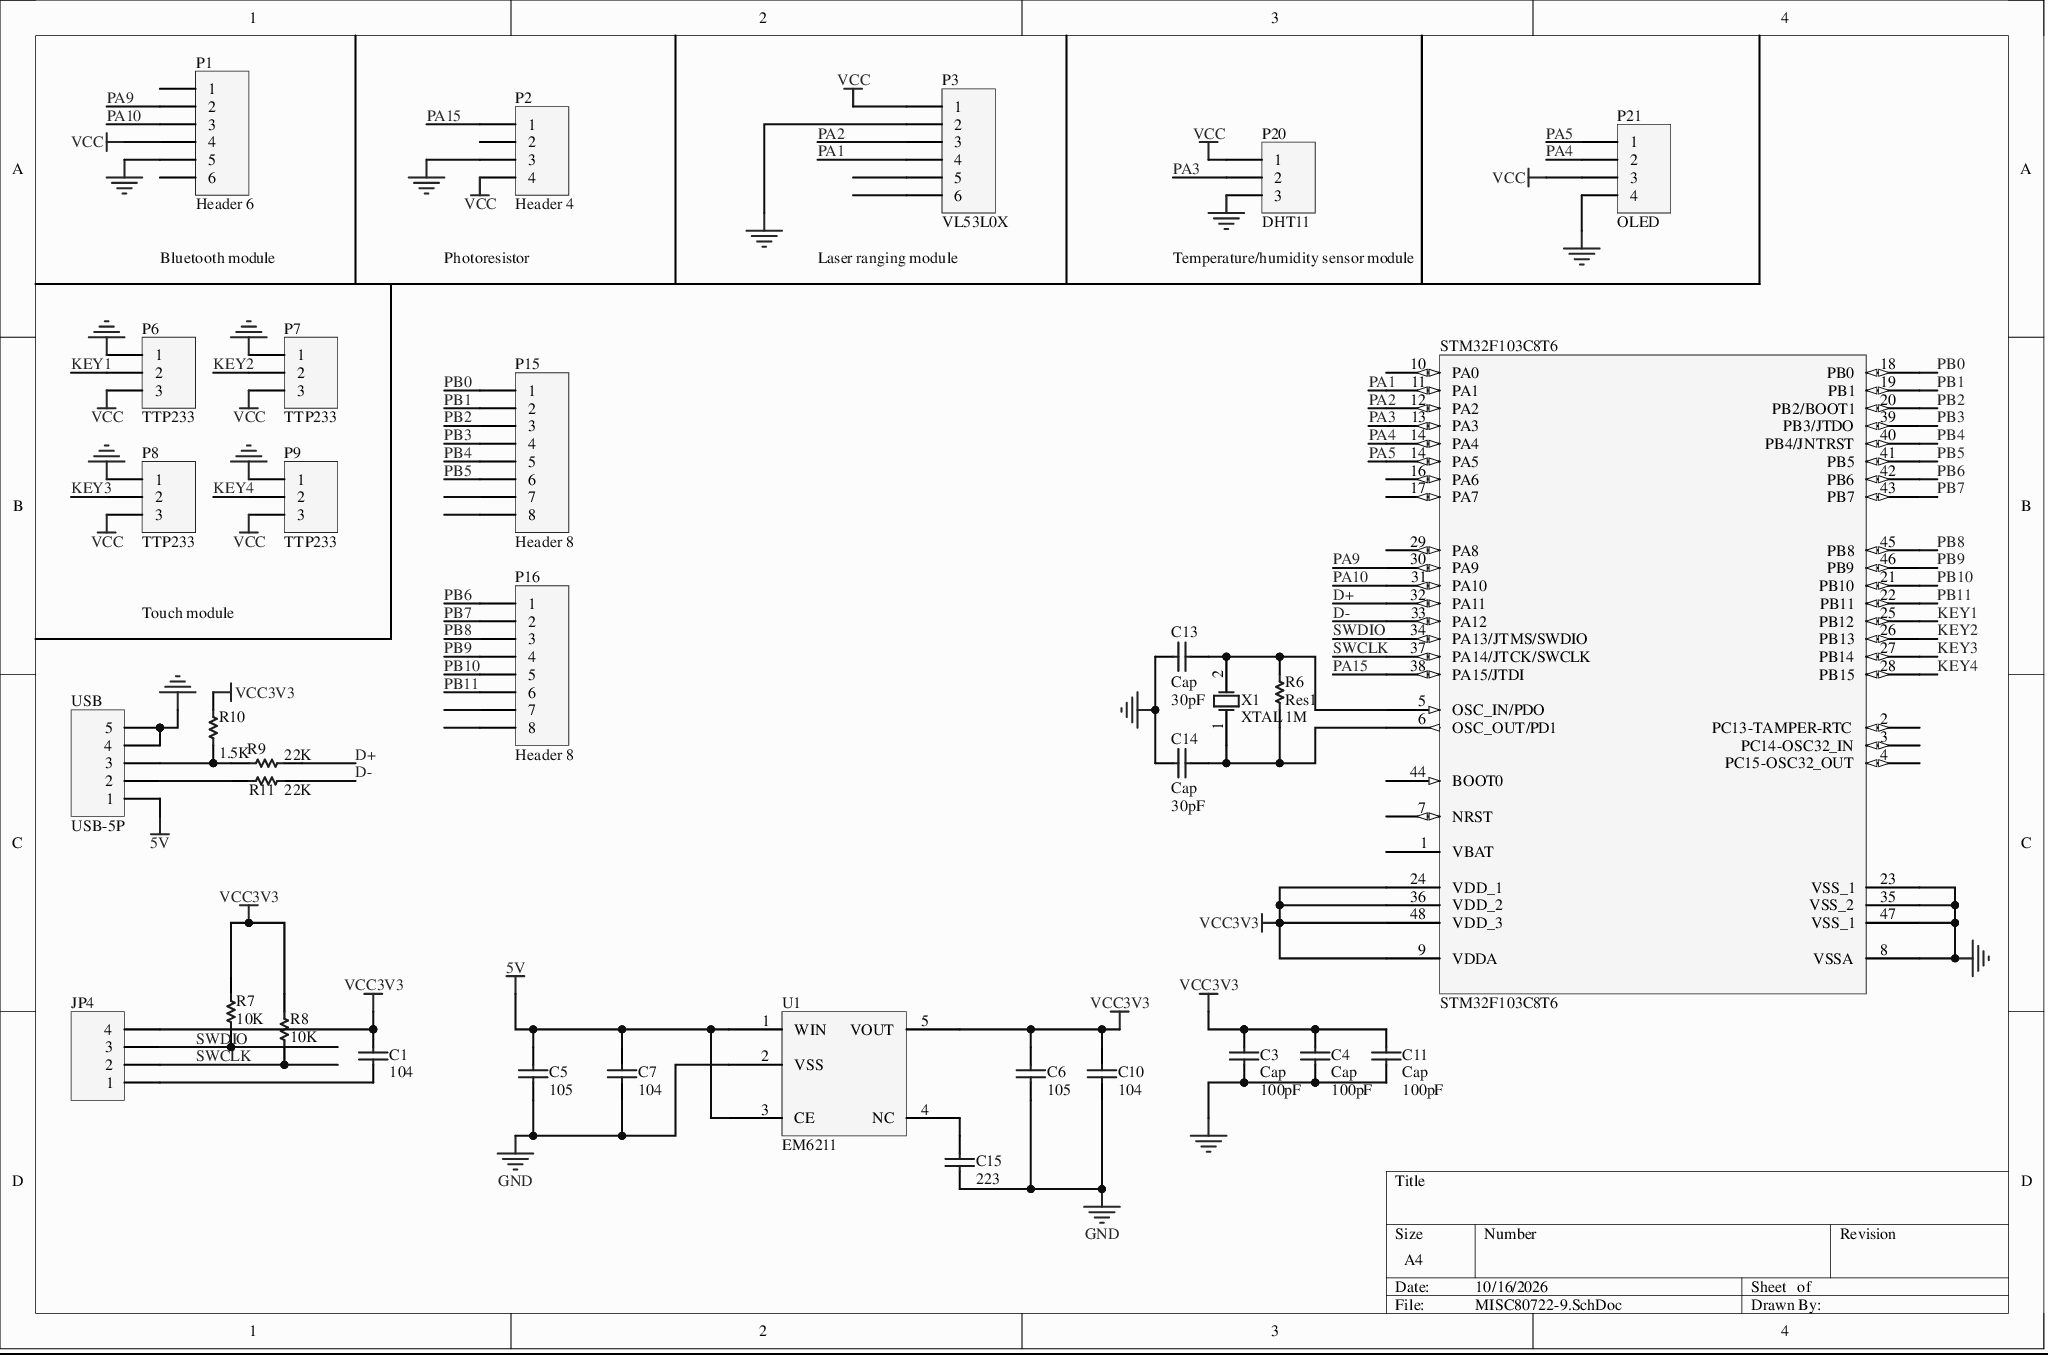
[diagram p0: MISC80722-9.SchDoc]
# Altium project MISC80722-4.PrjPcb
1 sheet, 33 parts. Net scope: global (net labels, ports and power ports of the same name join across sheets).
Board file: MISC80722.PcbDoc

## Sheet MISC80722-9.SchDoc
size A4; SheetNumber: 1; SheetTotal: 1

### Parts
C1  104  [RAD-0.3]
C3  Cap  value 100pF  [RAD-0.3]
C4  Cap  value 100pF  [RAD-0.3]
C5  105  [RAD-0.3]
C6  105  [RAD-0.3]
C7  104  [RAD-0.3]
C10  104  [RAD-0.3]
C11  Cap  value 100pF  [RAD-0.3]
C13  Cap  value 30pF  [RAD-0.3]
C14  Cap  value 30pF  [RAD-0.3]
C15  223  [RAD-0.3]
JP4  Header 4  [HDR1X4]  (value not drawn)
P1  Header 6  [HDR1X6]
P2  Header 4  [HDR1X4]
P3  VL53L0X  [HDR1X6]
P6  TTP233  [HDR1X3]
P7  TTP233  [HDR1X3]
P8  TTP233  [HDR1X3]
P9  TTP233  [HDR1X3]
P15  Header 8  [HDR1X8]
P16  Header 8  [HDR1X8]
P20  DHT11  [HDR1X3]
P21  OLED  [HDR1X4]
R6  Res1  value 1M  [AXIAL-0.3]
R7  value 10K  [AXIAL-0.3]  (hidden comment: Res1)
R8  value 10K  [AXIAL-0.3]  (hidden comment: Res1)
R9  value 22K  [AXIAL-0.3]  (hidden comment: Res1)
R10  value 1.5K  [AXIAL-0.3]  (hidden comment: Res1)
R11  value 22K  [AXIAL-0.3]  (hidden comment: Res1)
STM32F103C8T6  STM32F103C8T6  [PCBComponent_1]
U1  EM6211  [ME6211C28M5G]
USB  USB-5P  [HDR1X5]
X1  XTAL  [R38]

### Nets
5V: C5.2 C7.2 U1.1(WIN) U1.3(CE) USB.1
GND: C3.1 C4.1 C5.1 C6.1 C7.1 C10.1 C11.1 C13.2 C14.2 C15.1 P1.5 P2.3 P3.2 P6.1 P7.1 P8.1 P9.1 P20.3 P21.4 STM32F103C8T6.8(VSSA) STM32F103C8T6.23(VSS_1) STM32F103C8T6.35(VSS_2) STM32F103C8T6.47(VSS_1) U1.2(VSS) USB.4 USB.5
VCC: P1.4 P2.4 P3.1 P6.3 P7.3 P8.3 P9.3 P20.1 P21.3
VCC3V3: C1.2 C3.2 C4.2 C6.2 C10.2 C11.2 JP4.4 R7.1 R8.1 R10.2 STM32F103C8T6.9(VDDA) STM32F103C8T6.24(VDD_1) STM32F103C8T6.36(VDD_2) STM32F103C8T6.48(VDD_3) U1.5(VOUT)
D+: R9.1 STM32F103C8T6.32(PA11)
D-: R11.1 STM32F103C8T6.33(PA12)
KEY1: P6.2 STM32F103C8T6.25(PB12)
KEY2: P7.2 STM32F103C8T6.26(PB13)
KEY3: P8.2 STM32F103C8T6.27(PB14)
KEY4: P9.2 STM32F103C8T6.28(PB15)
PA1: P3.4 STM32F103C8T6.11(PA1)
PA2: P3.3 STM32F103C8T6.12(PA2)
PA3: P20.2 STM32F103C8T6.13(PA3)
PA4: P21.2 STM32F103C8T6.14(PA4)
PA5: P21.1 STM32F103C8T6.14(PA5)
PA9: P1.2 STM32F103C8T6.30(PA9)
PA10: P1.3 STM32F103C8T6.31(PA10)
PA15: P2.1 STM32F103C8T6.38(PA15/JTDI)
PB0: P15.1 STM32F103C8T6.18(PB0)
PB1: P15.2 STM32F103C8T6.19(PB1)
PB2: P15.3 STM32F103C8T6.20(PB2/BOOT1)
PB3: P15.4 STM32F103C8T6.39(PB3/JTDO)
PB4: P15.5 STM32F103C8T6.40(PB4/JNTRST)
PB5: P15.6 STM32F103C8T6.41(PB5)
PB6: P16.1 STM32F103C8T6.42(PB6)
PB7: P16.2 STM32F103C8T6.43(PB7)
PB8: P16.3 STM32F103C8T6.45(PB8)
PB9: P16.4 STM32F103C8T6.46(PB9)
PB10: P16.5 STM32F103C8T6.21(PB10)
PB11: P16.6 STM32F103C8T6.22(PB11)
SWCLK: JP4.2 R8.2 STM32F103C8T6.37(PA14/JTCK/SWCLK)
SWDIO: JP4.3 R7.2 STM32F103C8T6.34(PA13/JTMS/SWDIO)
NetC1_1: C1.1 JP4.1
NetC13_1: C13.1 R6.2 STM32F103C8T6.5(OSC_IN/PDO) X1.2(OSC2)
NetC14_1: C14.1 R6.1 STM32F103C8T6.6(OSC_OUT/PD1) X1.1(OSC1)
NetC15_2: C15.2 U1.4(NC)
NetR9_2: R9.2 R10.1 USB.3
NetR11_2: R11.2 USB.2

Not connected (* = marked no-connect by the designer): P1 1* 6*; P2 2*; P3 5* 6*; P15 7* 8*; P16 7* 8*; STM32F103C8T6 1(VBAT) 2(PC13-TAMPER-RTC) 3(PC14-OSC32_IN) 4(PC15-OSC32_OUT) 7(NRST) 10(PA0) 16(PA6) 17(PA7) 29(PA8) 44(BOOT0)

### Notes on the sheet
- Bluetooth module
- Photoresistor
- (near P3) Laser ranging module
- (near P20) Temperature/humidity sensor module
- Touch module

### Library data of the parts
C1 C5-C7 C10 C15 = Cap: Capacitor; Value: 100pF; Published: 8-Jun-2000; LatestRevisionDate: 17-Jul-2002; LatestRevisionNote: Re-released for DXP Platform.; PackageReference: RAD-0.3; PackageDescription: Radial Cap, Thru-Hole; 2 Leads; 0.3 in Pin Spacing; Publisher: Altium Limited
C3 C4 C11 C13 C14 = Cap: Capacitor; Published: 8-Jun-2000; LatestRevisionDate: 17-Jul-2002; LatestRevisionNote: Re-released for DXP Platform.; PackageReference: RAD-0.3; PackageDescription: Radial Cap, Thru-Hole; 2 Leads; 0.3 in Pin Spacing; Publisher: Altium Limited
JP4 P2 P21 = Header 4: Header, 4-Pin; LatestRevisionDate: 17-Jul-2002; LatestRevisionNote: Re-released for DXP Platform.; Publisher: Altium Limited
P1 P3 = Header 6: Header, 6-Pin; LatestRevisionDate: 17-Jul-2002; LatestRevisionNote: Re-released for DXP Platform.; Publisher: Altium Limited
P6-P9 P20 = Header 3: Header, 3-Pin; LatestRevisionDate: 17-Jul-2002; LatestRevisionNote: Re-released for DXP Platform.; Publisher: Altium Limited
P15 P16 = Header 8: Header, 8-Pin; LatestRevisionDate: 17-Jul-2002; LatestRevisionNote: Re-released for DXP Platform.; Publisher: Altium Limited
R6-R11 = Res1: Resistor; Published: 8-Jun-2000; LatestRevisionDate: 17-Jul-2002; LatestRevisionNote: Re-released for DXP Platform.; PackageReference: AXIAL-0.3; PackageDescription: Axial Device, Thru-Hole; 2 Leads; 0.3 in Pin Spacing; Publisher: Altium Limited
STM32F103C8T6 = Component_1
USB = Header 5: Header, 5-Pin; LatestRevisionDate: 17-Jul-2002; LatestRevisionNote: Re-released for DXP Platform.; Publisher: Altium Limited
X1 = XTAL: Crystal Oscillator; Published: 8-Jun-2000; LatestRevisionDate: 17-Jul-2002; LatestRevisionNote: Re-released for DXP Platform.; PackageReference: R38; PackageDescription: Crystal, Thru-Hole; 2 Leads; Body 3.1 x 8.2 mm (Dia.xH); Publisher: Altium Limited